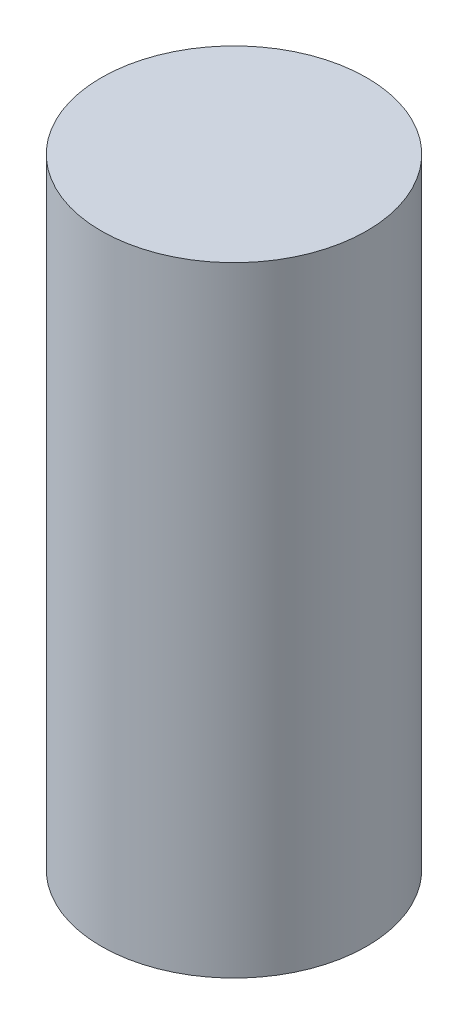
SolidWorks part; units mm, degrees
ref_plane "Front Plane" through (0, 0, 0) normal (0, 0, 1) x (1, 0, 0)
ref_plane "Top Plane" through (0, 0, 0) normal (0, 1, 0) x (1, 0, 0)
ref_plane "Right Plane" through (0, 0, 0) normal (1, 0, 0) x (0, 0, -1)
sketch "Sketch1" plane through (0, 0, 0) normal (0, 1, 0) x (1, 0, 0)
  circle A0 centre (0, 0) radius 15
  dimension "D1" = 30
extrude "Boss-Extrude1" add sketch "Sketch1" along normal mid plane 70
sketch "Sketch2" plane through (0, -35, 0) normal (0, -1, 0) x (1, 0, 0)
  circle A0 centre (0, 0) radius 11.7291
hole_wizard "M20 Tapped Hole1" positions "3DSketch2" profile "Sketch4" tap size "M20" standard "GB"
sketch3d "3DSketch2"
  point P0 (0, -35, 0)
sketch "Sketch4" plane through (0, -35, 0) normal (1, 0, 0) x (0, 0, -1)
  line L0 (0, 0) -> (0, 57.7575)
  line L1 (0, 57.7575) -> (8.75, 52.5)
  line L2 (8.75, 52.5) -> (8.75, 0)
  line L5 (8.75, 0) -> (0, 0)
  line L10 (0, 57.7575) -> (-8.75, 52.5) construction
  line L11 (0, -6.35) -> (0, 107.95) construction
  dimension "螺纹孔钻头直径" = 17.5
  dimension "螺纹孔钻头深度" = 52.5
  dimension "导头角度" = 118
cosmetic thread "Hole Cosmetic Thread1" parameters "D1"=40, "D2"=20
ref_plane "Plane1" through (0, 5, 0) normal (0, -1, 0) x (-1, 0, 0)
